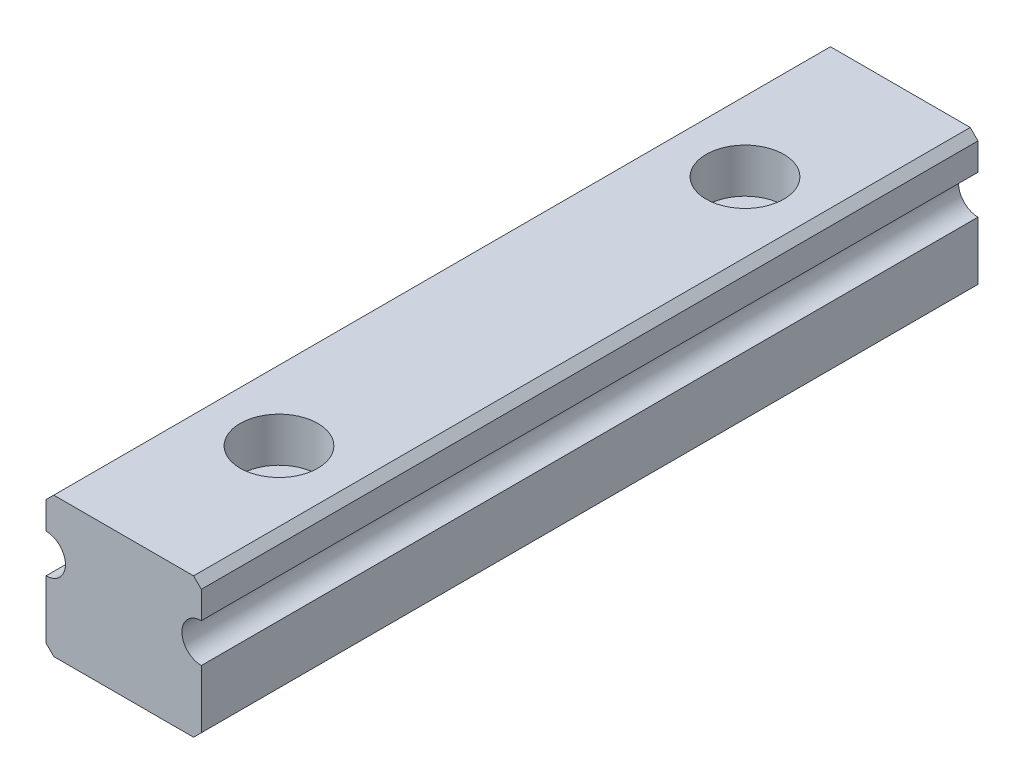
SolidWorks part; units mm, degrees
ref_plane "Front Plane" through (0, 0, 0) normal (0, 0, 1) x (1, 0, 0)
ref_plane "Top Plane" through (0, 0, 0) normal (0, 1, 0) x (1, 0, 0)
ref_plane "Right Plane" through (0, 0, 0) normal (1, 0, 0) x (0, 0, -1)
sketch "Sketch1" plane through (0, 0, 0) normal (0, 0, 1) x (1, 0, 0)
  line L0 (0, 13.5) -> (0, 17)
  line L1 (1, 0) -> (19, 0)
  line L2 (0, 1) -> (0, 8.5)
  line L3 (1, 18) -> (19, 18)
  line L4 (20, 1) -> (20, 8.5)
  line L5 (20, 13.5) -> (20, 17)
  line L6 (0, 17) -> (1, 18)
  line L7 (19, 18) -> (20, 17)
  line L8 (19, 0) -> (20, 1)
  line L9 (0, 1) -> (1, 0)
  arc A0 (0, 8.5) -> (0, 13.5) centre (0, 11) ccw
  arc A1 (20, 13.5) -> (20, 8.5) centre (20, 11) ccw
  point P0 (0, 0)
  point P1 (20, 18)
  point P2 (0, 18)
  point P3 (20, 0)
  dimension "D3" = 5
  dimension "D1" = 20
  dimension "D2" = 18
  dimension "D4" = 11
extrude "Extrude1" add sketch "Sketch1" along normal blind 100
hole_wizard "Hole size per socket head cap screw type 1" positions "3DSketch1" profile "Sketch3" counterbore size "M5" standard "GB" end condition through all
sketch3d "3DSketch1"
  line L0 (19, 18, 0) -> (1, 18, 0) construction
  point P1 (10, 18, 20)
  point P3 (10, 18, 80)
  dimension "D1" = 20
  dimension "D2" = 60
  dimension "D6" = 10
sketch "Sketch3" plane through (10, 18, 20) normal (1, 0, 0) x (0, 0, 1)
  line L0 (0, 0) -> (0, 18)
  line L1 (0, 18) -> (2.75, 18)
  line L3 (2.75, 18) -> (2.75, 5.7)
  line L4 (2.75, 5.7) -> (5, 5.7)
  line L5 (5, 5.7) -> (5, 0)
  line L7 (5, 0) -> (0, 0)
  line L11 (0, -6.35) -> (0, 107.95) construction
  dimension "通孔孔直径" = 5.5
  dimension "通孔孔深度" = 18
  dimension "柱形沉头孔直径" = 10
  dimension "柱形沉头孔深度" = 5.7
